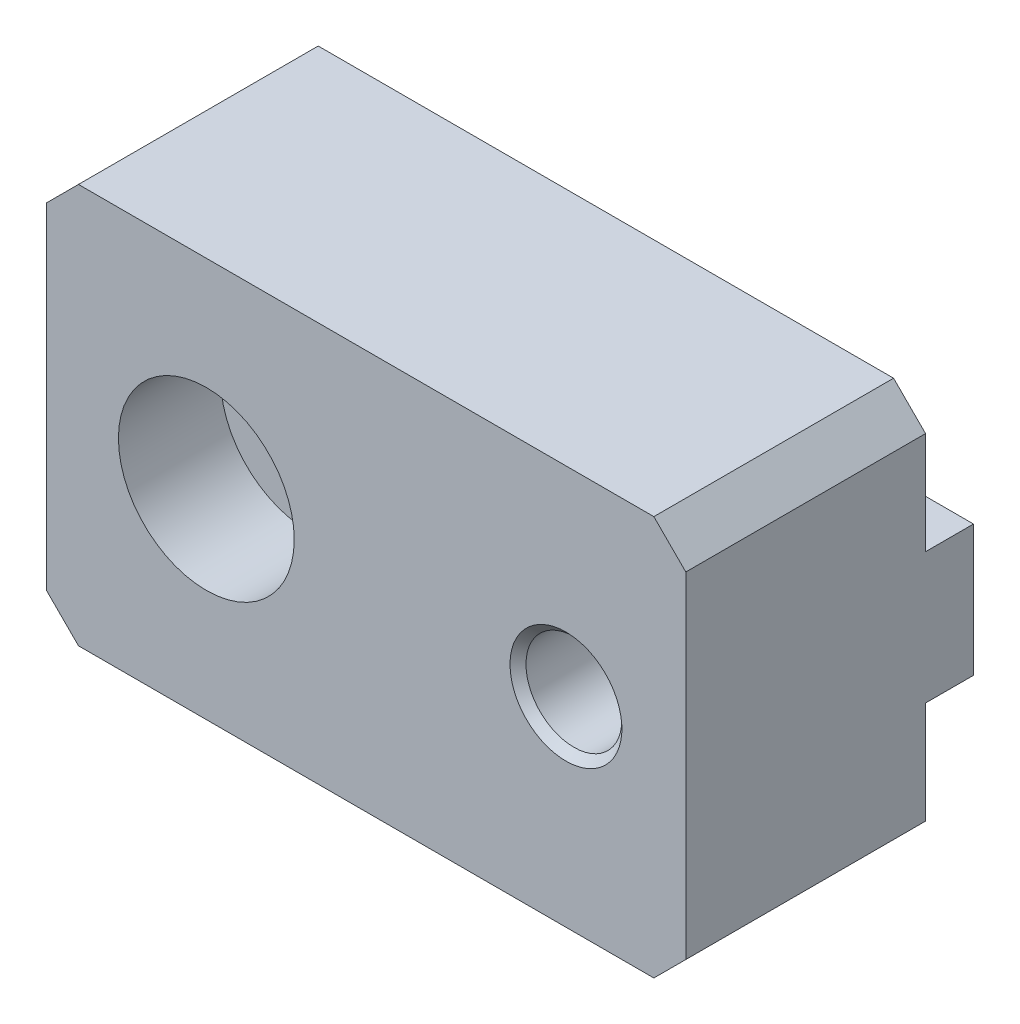
SolidWorks part; units mm, degrees
ref_plane "前视基准面" through (0, 0, 0) normal (0, 0, 1) x (1, 0, 0)
ref_plane "上视基准面" through (0, 0, 0) normal (0, 1, 0) x (1, 0, 0)
ref_plane "右视基准面" through (0, 0, 0) normal (1, 0, 0) x (0, 0, -1)
sketch "草图1" plane through (0, 0, 0) normal (0, 0, 1) x (1, 0, 0)
  line L1 (0, 0) -> (40, 0)
  line L2 (0, 0) -> (0, 25)
  line L3 (0, 25) -> (40, 25)
  line L4 (40, 0) -> (40, 25)
  dimension "D1" = 40
  dimension "D2" = 25
extrude "凸台-拉伸1" add sketch "草图1" along normal blind 15
sketch "草图9" plane through (0, 0, 0) normal (0, 0, -1) x (-1, 0, 0)
  line L0 (0, 12.5) -> (-40, 12.5) construction
  line L1 (-40, 8.4) -> (0, 8.4)
  line L2 (-40, 8.4) -> (-40, 16.6)
  line L3 (-40, 16.6) -> (0, 16.6)
  line L4 (0, 8.4) -> (0, 16.6)
  line L5 (0, 25) -> (0, 0) construction
  line L6 (-40, 0) -> (-40, 25) construction
  dimension "D1" = 8.2
extrude "凸台-拉伸3" add sketch "草图9" along normal blind 3
hole_wizard "M6 六角凹头螺钉的柱形沉头孔2" positions "草图11" profile "草图10" counterbore size "M6" standard "ISO" end condition through all
sketch "草图11" plane through (0, 0, 15) normal (0, 0, 1) x (1, 0, 0)
  line L0 (40, 12.5) -> (0, 12.5) construction
  line L1 (40, 0) -> (40, 25) construction
  line L2 (0, 25) -> (0, 0) construction
  point P0 (10, 12.5)
  dimension "D1" = 10
sketch "草图10" plane through (10, 12.5, 15) normal (1, 0, 0) x (0, -1, 0)
  line L0 (0, 0) -> (0, 18)
  line L1 (0, 18) -> (3.3, 18)
  line L3 (3.3, 18) -> (3.3, 6.4)
  line L4 (3.3, 6.4) -> (5.5, 6.4)
  line L5 (5.5, 6.4) -> (5.5, 0)
  line L7 (5.5, 0) -> (0, 0)
  line L11 (0, -6.35) -> (0, 107.95) construction
  dimension "通孔孔直径" = 6.6
  dimension "通孔孔深度" = 18
  dimension "柱形沉头孔直径" = 11
  dimension "柱形沉头孔深度" = 6.4
sketch "草图12" plane through (0, 0, 15) normal (0, 0, 1) x (1, 0, 0)
  line L0 (40, 12.5) -> (0, 12.5) construction
  line L1 (40, 0) -> (40, 25) construction
  line L2 (0, 25) -> (0, 0) construction
  circle A0 centre (32.5, 12.5) radius 3
  dimension "D2" = 6
  dimension "D1" = 7.5
extrude "切除-拉伸3" cut sketch "草图12" against normal through all
chamfer "倒角2" distance 0.5 angle 45 1 edges at (35.5, 12.5, 15)
chamfer "倒角3" distance 2 angle 45 4 edges at (40, 0, 7.5) (0, 0, 7.5) (0, 25, 7.5) (40, 25, 7.5)
